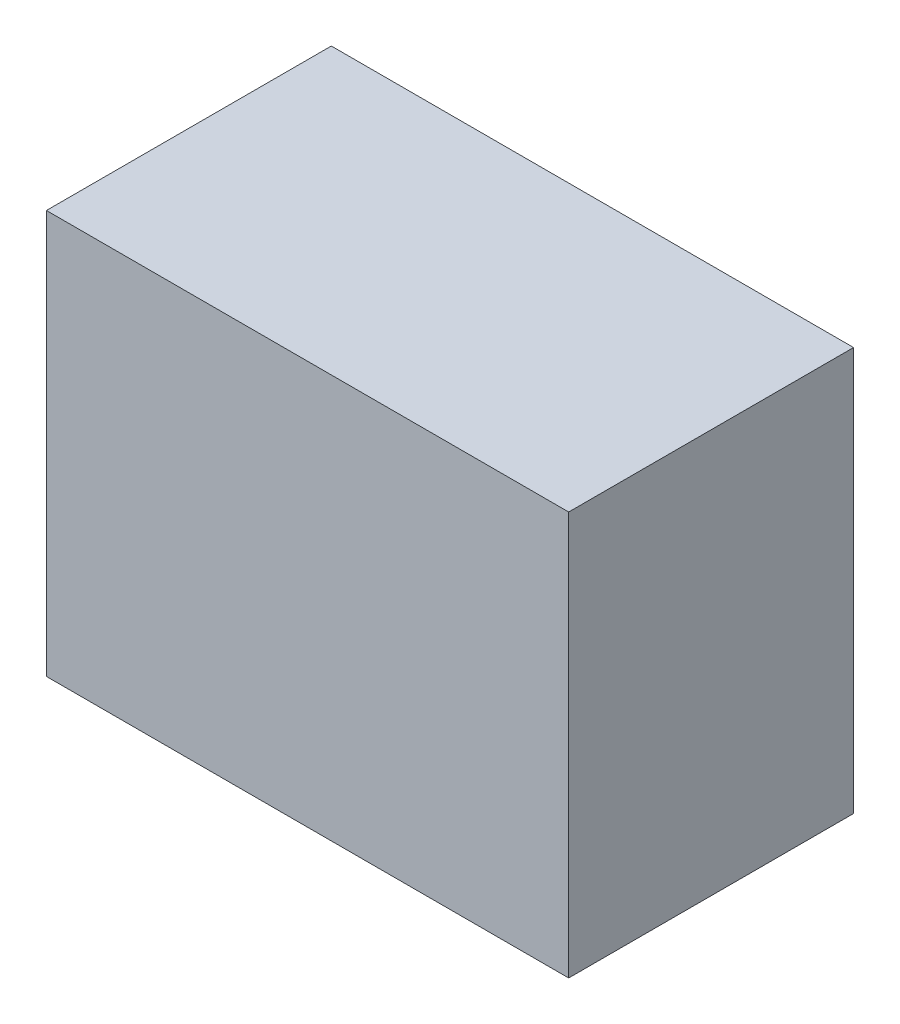
SolidWorks part; units mm, degrees
material "普通碳钢"
ref_plane "Front Plane" through (0, 0, 0) normal (0, 0, 1) x (1, 0, 0)
ref_plane "Top Plane" through (0, 0, 0) normal (0, 1, 0) x (1, 0, 0)
ref_plane "Right Plane" through (0, 0, 0) normal (1, 0, 0) x (0, 0, -1)
sketch "Sketch1" plane through (0, 0, 0) normal (0, 0, 1) x (1, 0, 0)
  line L1 (0, 0) -> (1100, 0)
  line L2 (0, 0) -> (0, 850)
  line L3 (0, 850) -> (1100, 850)
  line L4 (1100, 0) -> (1100, 850)
  dimension "D1" = 1100
  dimension "D2" = 850
extrude "Boss-Extrude1" add sketch "Sketch1" along normal blind 600
